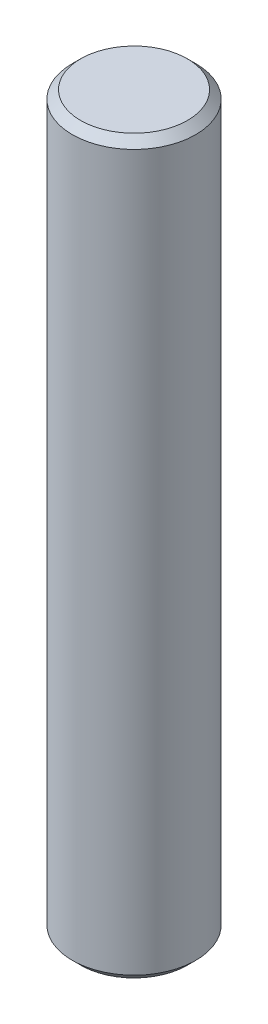
SolidWorks part; units mm, degrees
ref_plane "Front Plane" through (0, 0, 0) normal (0, 0, 1) x (1, 0, 0)
ref_plane "Top Plane" through (0, 0, 0) normal (0, 1, 0) x (1, 0, 0)
ref_plane "Right Plane" through (0, 0, 0) normal (1, 0, 0) x (0, 0, -1)
sketch "Sketch1" plane through (0, 0, 0) normal (0, 0, 1) x (1, 0, 0)
  line L0 (0, 0) -> (0, 49.4999) construction
  line L1 (0, 0) -> (15, 0)
  line L2 (15, 0) -> (15, 178)
  line L3 (15, 178) -> (0, 178)
  line L4 (0, 178) -> (0, 0)
  dimension "D1" = 178
revolve "Revolve1" add sketch "Sketch1" angle 360 about L0
chamfer "Chamfer1" distance 2 angle 45 2 edges at (0, 0, -15) (0, 178, -15)
